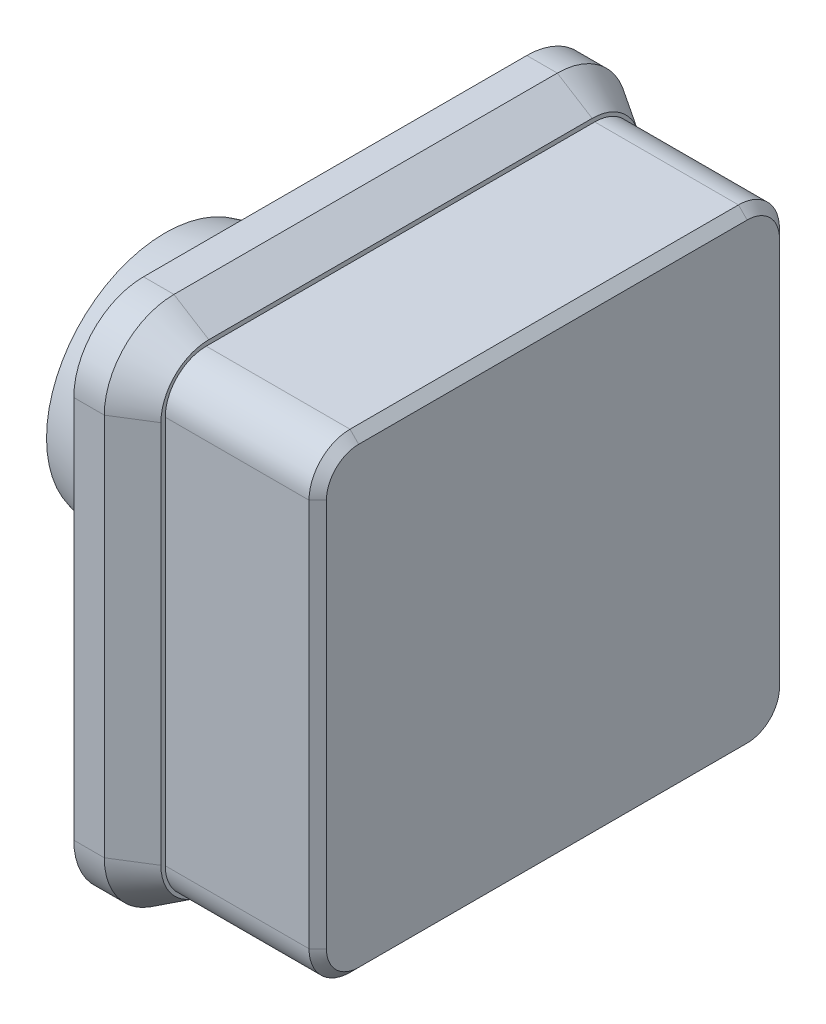
from build123d import *
from OCP.BRepFilletAPI import BRepFilletAPI_MakeChamfer

# Parameters (mm, degrees)
SKETCH1_W           = 10
SKETCH1_H           = 35
BOSS_EXTRUDE1_DEPTH = 15
CHAMFER1_SIZE       = 8
CHAMFER1_SIZE2      = 5
BOSS_EXTRUDE2_DEPTH = 35
CHAMFER2_SIZE       = 2
CHAMFER3_SIZE       = 1
CHAMFER3_SIZE2      = 1.414213562


with BuildPart() as part:
    # Sketch1 → Revolve1 (revolve)
    with BuildSketch(Plane(origin=(0, 0, 0), x_dir=(1, 0, 0), z_dir=(0, 1, 0)), mode=Mode.PRIVATE) as revolve1_sk:
        with Locations((35, 17.5)):
            Rectangle(SKETCH1_W, SKETCH1_H)
        Polygon((0, 0), (30, 0), (30, 35), (0, 26.961524227), align=None)
    revolve(revolve1_sk.sketch.rotate(Axis((0, 0, 0), (1, 0, 0)), 180), axis=Axis((0, 0, 0), (1, 0, 0)))

    # Sketch2 → Boss-Extrude1 (add)
    with BuildSketch(Plane(origin=(40, 0, 0), x_dir=(0, 0, -1), z_dir=(1, 0, 0))):
        with BuildLine():
            Line((-44, -60), (44, -60))
            ThreePointArc((44, -60), (55.313708499, -55.313708499), (60, -44))
            Line((60, -44), (60, 44))
            ThreePointArc((60, 44), (55.313708499, 55.313708499), (44, 60))
            Line((44, 60), (-44, 60))
            ThreePointArc((-44, 60), (-55.313708499, 55.313708499), (-60, 44))
            Line((-60, 44), (-60, -44))
            ThreePointArc((-60, -44), (-55.313708499, -55.313708499), (-44, -60))
        make_face()
    extrude(amount=BOSS_EXTRUDE1_DEPTH)

    # Chamfer1: one chamfer whose edges measure the first distance from different faces: ONE call of the kernel's chamfer builder (chamfer() names one face for all edges)
    chamfer1_edges_1 = [part.edges().sort_by_distance(p)[0] for p in [
        (55, -55.313708499, 55.313708499),
    ]]
    chamfer1_side_1 = [part.faces().sort_by_distance(p)[0] for p in [
        (47.5, -55.313708499, 55.313708499),
    ]]
    chamfer1_edges_2 = [part.edges().sort_by_distance(p)[0] for p in [
        (55, -60, 0),
    ]]
    chamfer1_side_2 = [part.faces().sort_by_distance(p)[0] for p in [
        (47.5, -60, 0),
    ]]
    chamfer1_edges_3 = [part.edges().sort_by_distance(p)[0] for p in [
        (55, -55.313708499, -55.313708499),
    ]]
    chamfer1_side_3 = [part.faces().sort_by_distance(p)[0] for p in [
        (47.5, -55.313708499, -55.313708499),
    ]]
    chamfer1_edges_4 = [part.edges().sort_by_distance(p)[0] for p in [
        (55, 0, -60),
    ]]
    chamfer1_side_4 = [part.faces().sort_by_distance(p)[0] for p in [
        (47.5, 0, -60),
    ]]
    chamfer1_edges_5 = [part.edges().sort_by_distance(p)[0] for p in [
        (55, 55.313708499, -55.313708499),
    ]]
    chamfer1_side_5 = [part.faces().sort_by_distance(p)[0] for p in [
        (47.5, 55.313708499, -55.313708499),
    ]]
    chamfer1_edges_6 = [part.edges().sort_by_distance(p)[0] for p in [
        (55, 60, 0),
    ]]
    chamfer1_side_6 = [part.faces().sort_by_distance(p)[0] for p in [
        (47.5, 60, 0),
    ]]
    chamfer1_edges_7 = [part.edges().sort_by_distance(p)[0] for p in [
        (55, 55.313708499, 55.313708499),
    ]]
    chamfer1_side_7 = [part.faces().sort_by_distance(p)[0] for p in [
        (47.5, 55.313708499, 55.313708499),
    ]]
    chamfer1_edges_8 = [part.edges().sort_by_distance(p)[0] for p in [
        (55, 0, 60),
    ]]
    chamfer1_side_8 = [part.faces().sort_by_distance(p)[0] for p in [
        (47.5, 0, 60),
    ]]
    chamfer1 = BRepFilletAPI_MakeChamfer(part.part.solid().wrapped)
    for e in chamfer1_edges_1:
        chamfer1.Add(CHAMFER1_SIZE, CHAMFER1_SIZE2, e.wrapped, chamfer1_side_1[0].wrapped)  # the first distance lies on this face
    for e in chamfer1_edges_2:
        chamfer1.Add(CHAMFER1_SIZE, CHAMFER1_SIZE2, e.wrapped, chamfer1_side_2[0].wrapped)  # the first distance lies on this face
    for e in chamfer1_edges_3:
        chamfer1.Add(CHAMFER1_SIZE, CHAMFER1_SIZE2, e.wrapped, chamfer1_side_3[0].wrapped)  # the first distance lies on this face
    for e in chamfer1_edges_4:
        chamfer1.Add(CHAMFER1_SIZE, CHAMFER1_SIZE2, e.wrapped, chamfer1_side_4[0].wrapped)  # the first distance lies on this face
    for e in chamfer1_edges_5:
        chamfer1.Add(CHAMFER1_SIZE, CHAMFER1_SIZE2, e.wrapped, chamfer1_side_5[0].wrapped)  # the first distance lies on this face
    for e in chamfer1_edges_6:
        chamfer1.Add(CHAMFER1_SIZE, CHAMFER1_SIZE2, e.wrapped, chamfer1_side_6[0].wrapped)  # the first distance lies on this face
    for e in chamfer1_edges_7:
        chamfer1.Add(CHAMFER1_SIZE, CHAMFER1_SIZE2, e.wrapped, chamfer1_side_7[0].wrapped)  # the first distance lies on this face
    for e in chamfer1_edges_8:
        chamfer1.Add(CHAMFER1_SIZE, CHAMFER1_SIZE2, e.wrapped, chamfer1_side_8[0].wrapped)  # the first distance lies on this face
    add(Compound.cast(chamfer1.Shape()), mode=Mode.REPLACE)

    # Sketch3 → Boss-Extrude2 (add)
    with BuildSketch(Plane(origin=(55, 0, 0), x_dir=(0, 0, -1), z_dir=(1, 0, 0))):
        with BuildLine():
            Line((-44.591144521, -54), (44.591144521, -54))
            ThreePointArc((44.591144521, -54), (51.244210033, -51.244210033), (54, -44.591144521))
            Line((54, -44.591144521), (54, 44.591144521))
            ThreePointArc((54, 44.591144521), (51.244210033, 51.244210033), (44.591144521, 54))
            Line((44.591144521, 54), (-44.591144521, 54))
            ThreePointArc((-44.591144521, 54), (-51.244210033, 51.244210033), (-54, 44.591144521))
            Line((-54, 44.591144521), (-54, -44.591144521))
            ThreePointArc((-54, -44.591144521), (-51.244210033, -51.244210033), (-44.591144521, -54))
        make_face()
    extrude(amount=BOSS_EXTRUDE2_DEPTH)

    # Chamfer2
    chamfer2_edges = [part.edges().sort_by_distance(p)[0] for p in [
        (90, 51.244210033, -51.244210033),
        (90, 54, 0),
        (90, 51.244210033, 51.244210033),
        (90, 0, 54),
        (90, -51.244210033, 51.244210033),
        (90, -54, 0),
        (90, -51.244210033, -51.244210033),
        (90, 0, -54),
    ]]
    chamfer(chamfer2_edges, length=CHAMFER2_SIZE)

    # Chamfer3
    chamfer3_edges = [part.edges().sort_by_distance(p)[0] for p in [
        (0, 0, -26.961524227),
    ]]
    chamfer3_side = [part.faces().sort_by_distance(p)[0] for p in [
        (15, 0, -30.980762114),
    ]]
    chamfer(chamfer3_edges, length=CHAMFER3_SIZE, length2=CHAMFER3_SIZE2, reference=chamfer3_side[0])


solid = part.part
